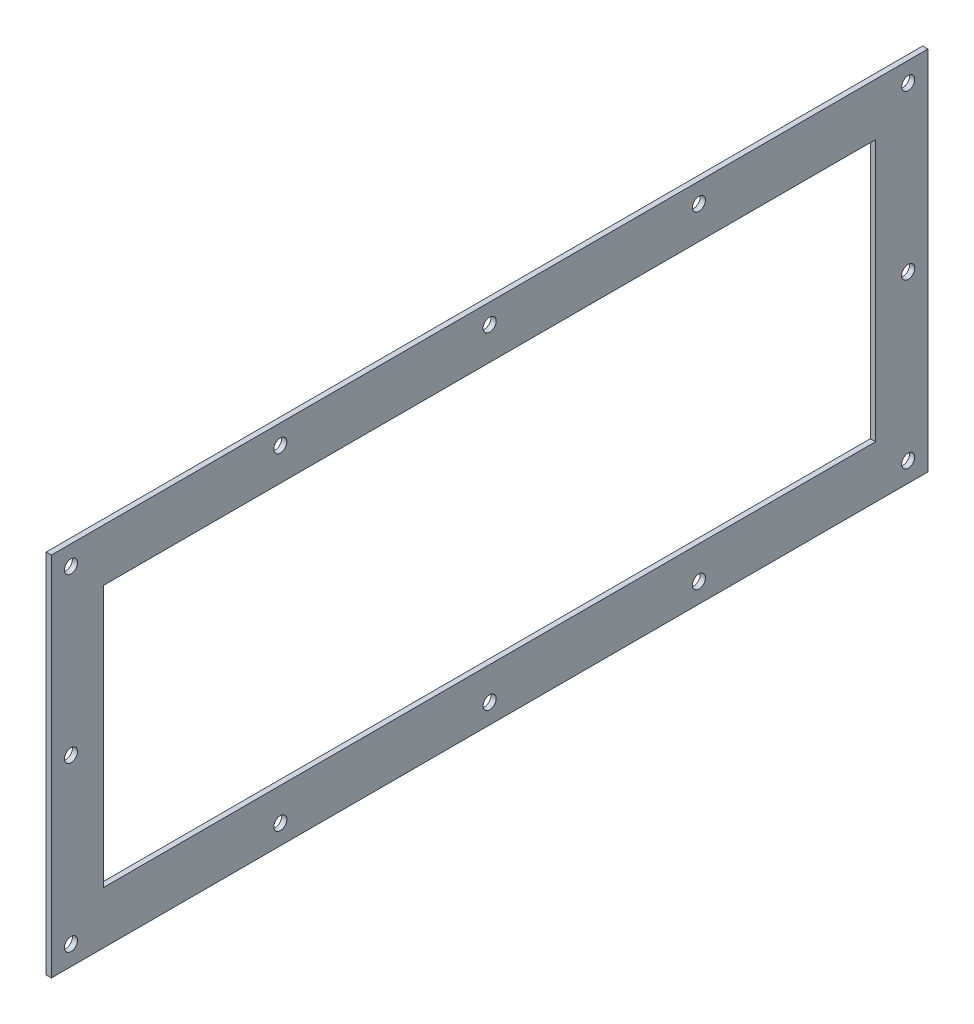
from build123d import *

# Parameters (mm, degrees)
SKETCH_1_W                  = 670
SKETCH_1_H                  = 280
SKETCH_1_W_2                = 590
SKETCH_1_H_2                = 200
EXTRUDE_1_DEPTH             = 4
HOLE_WIZARD_10_0_10_1_D     = 10
PATTERN_LINEAR_1_COUNT      = 5
PATTERN_LINEAR_1_PITCH      = 160
PATTERN_LINEAR_1_COUNT_DIR2 = 3
PATTERN_LINEAR_1_PITCH_DIR2 = 125


with BuildPart() as part:
    # 草图1 → 拉伸-薄壁1 (new body)
    with BuildSketch(Plane(origin=(0, 0, 0), x_dir=(0, 0, -1), z_dir=(1, 0, 0))):
        Rectangle(SKETCH_1_W, SKETCH_1_H)
        Rectangle(SKETCH_1_W_2, SKETCH_1_H_2, mode=Mode.SUBTRACT)
    extrude(amount=EXTRUDE_1_DEPTH)

    # Ø10.0 (10) 直径孔1 (through all)
    with Locations(Plane(origin=(4, 0, 0), x_dir=(0, 0, -1), z_dir=(1, 0, 0))):
        with Locations((-320, 125)):
            hole_wizard_10_0_10_1 = Hole(HOLE_WIZARD_10_0_10_1_D / 2)

    # 阵列(线性)1: Hole Wizard 10.0 _10_ _1 5 × 3, 3 skipped
    with Locations(*[(0, -j * PATTERN_LINEAR_1_PITCH_DIR2, -i * PATTERN_LINEAR_1_PITCH) for i in range(PATTERN_LINEAR_1_COUNT) for j in range(PATTERN_LINEAR_1_COUNT_DIR2) if (i, j) not in ((0, 0), (1, 1), (2, 1), (3, 1))]):
        add(hole_wizard_10_0_10_1, mode=Mode.SUBTRACT)


solid = part.part
